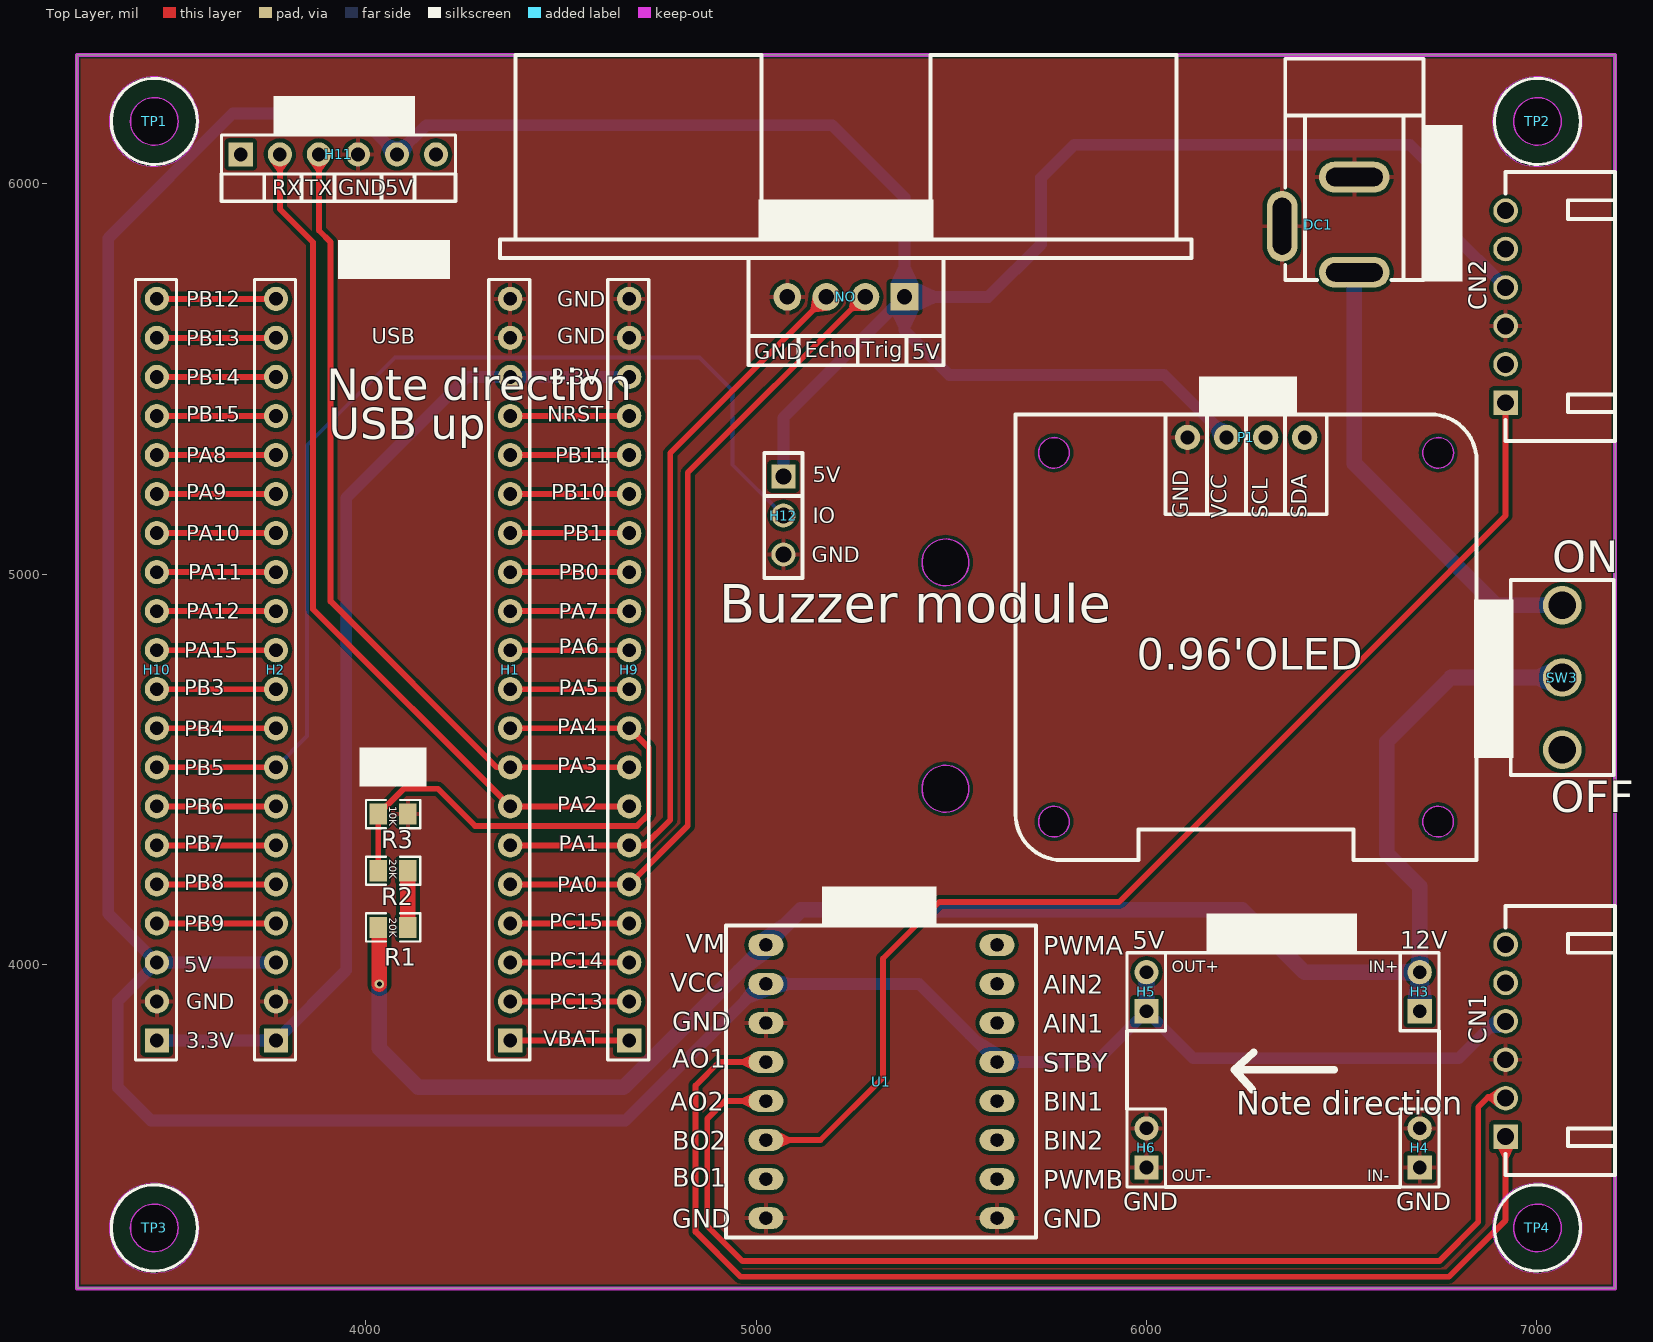
[diagram p0: Top Layer view]
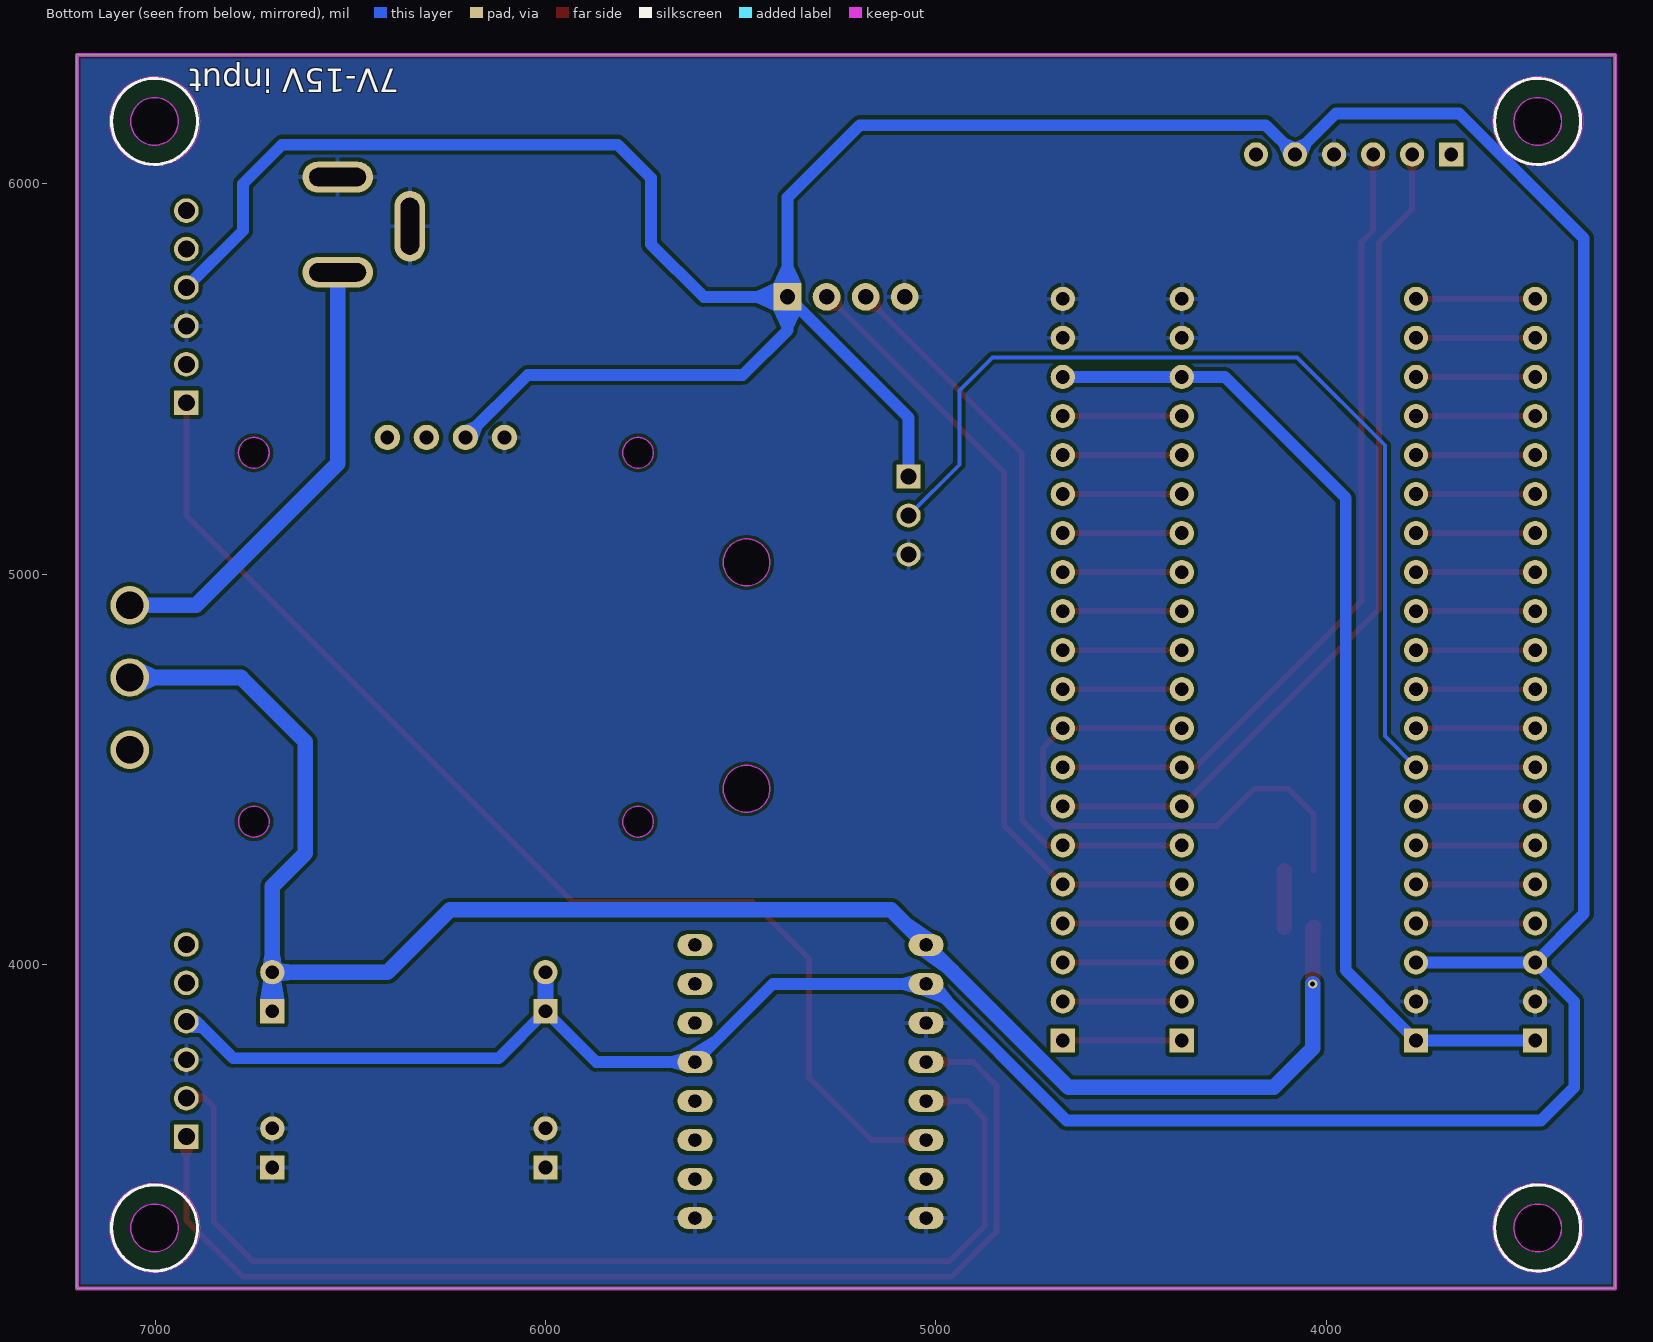
[diagram p1: Bottom Layer view, seen from below]
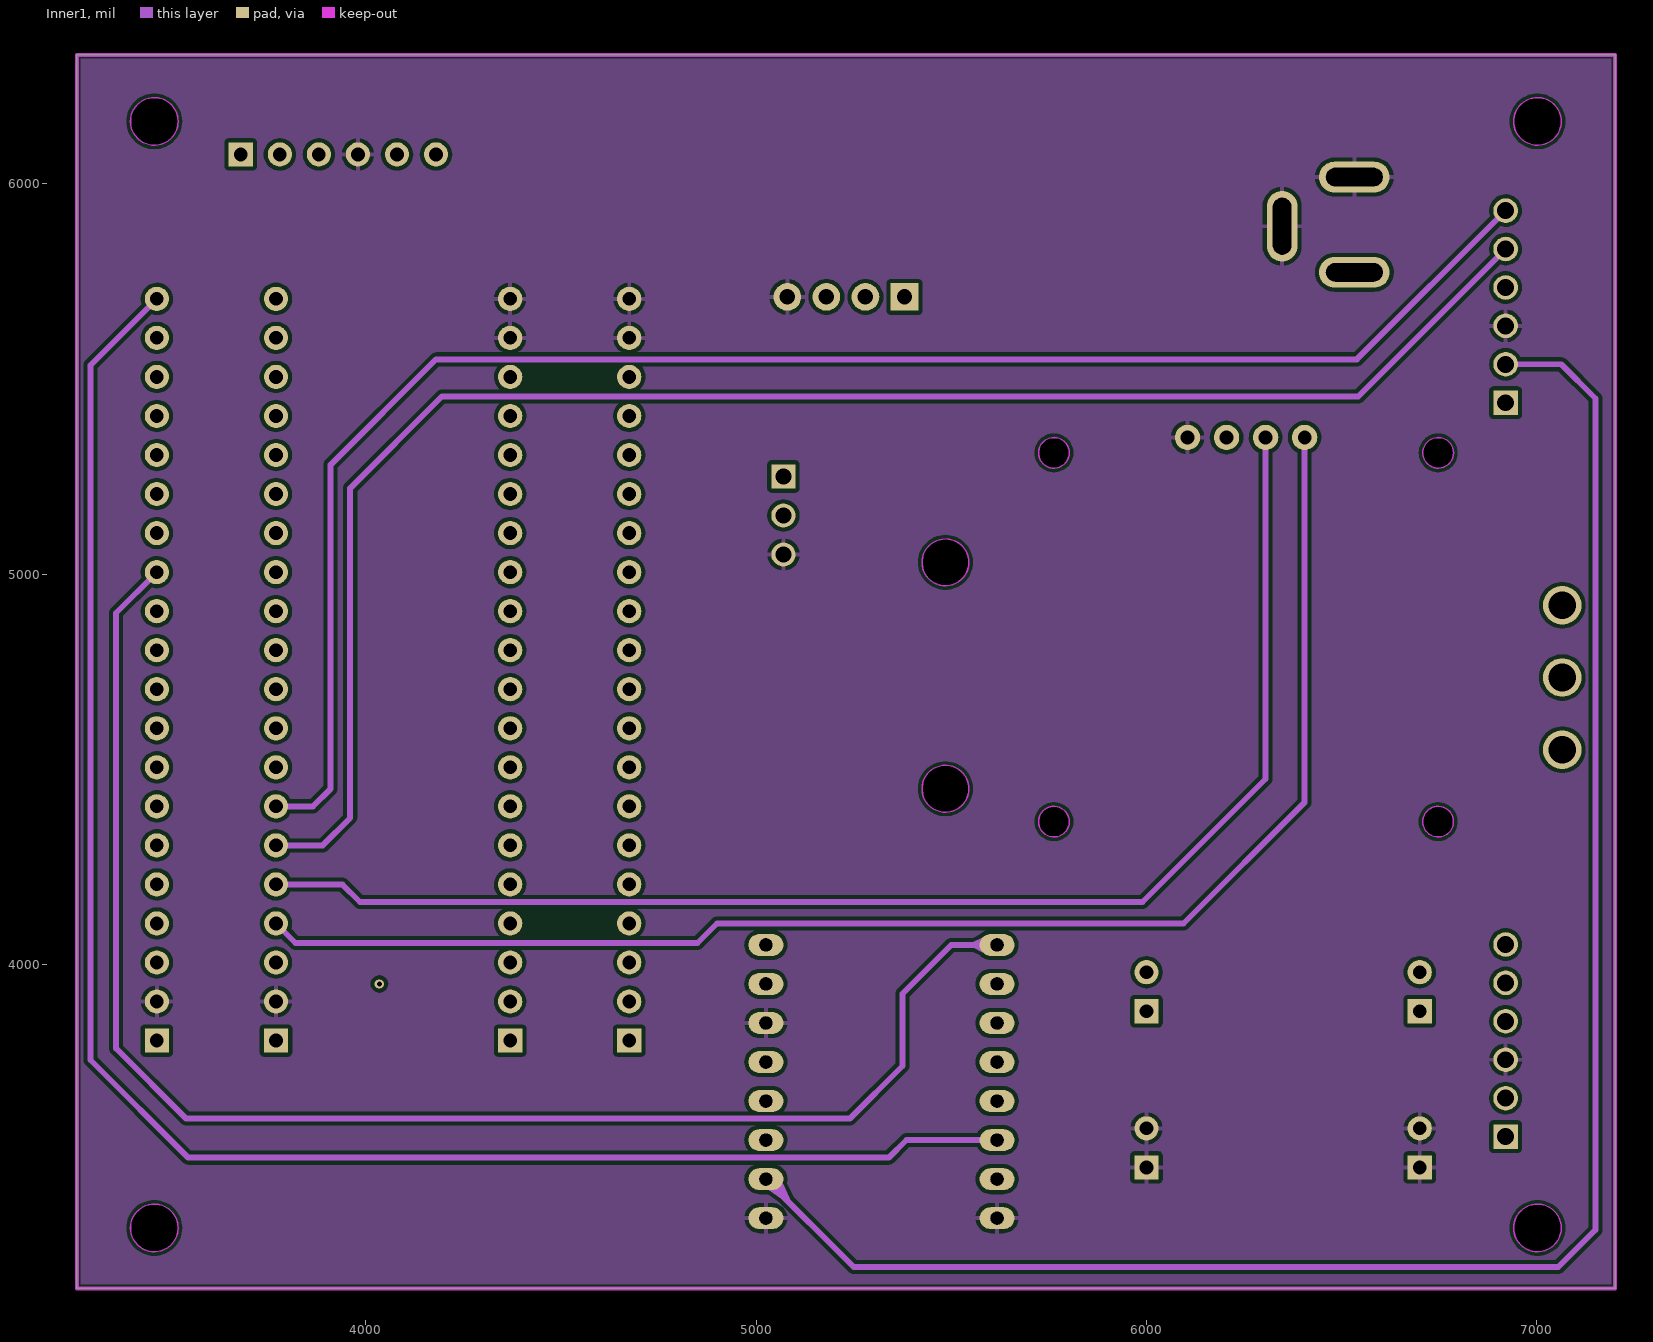
[diagram p2: Inner1]
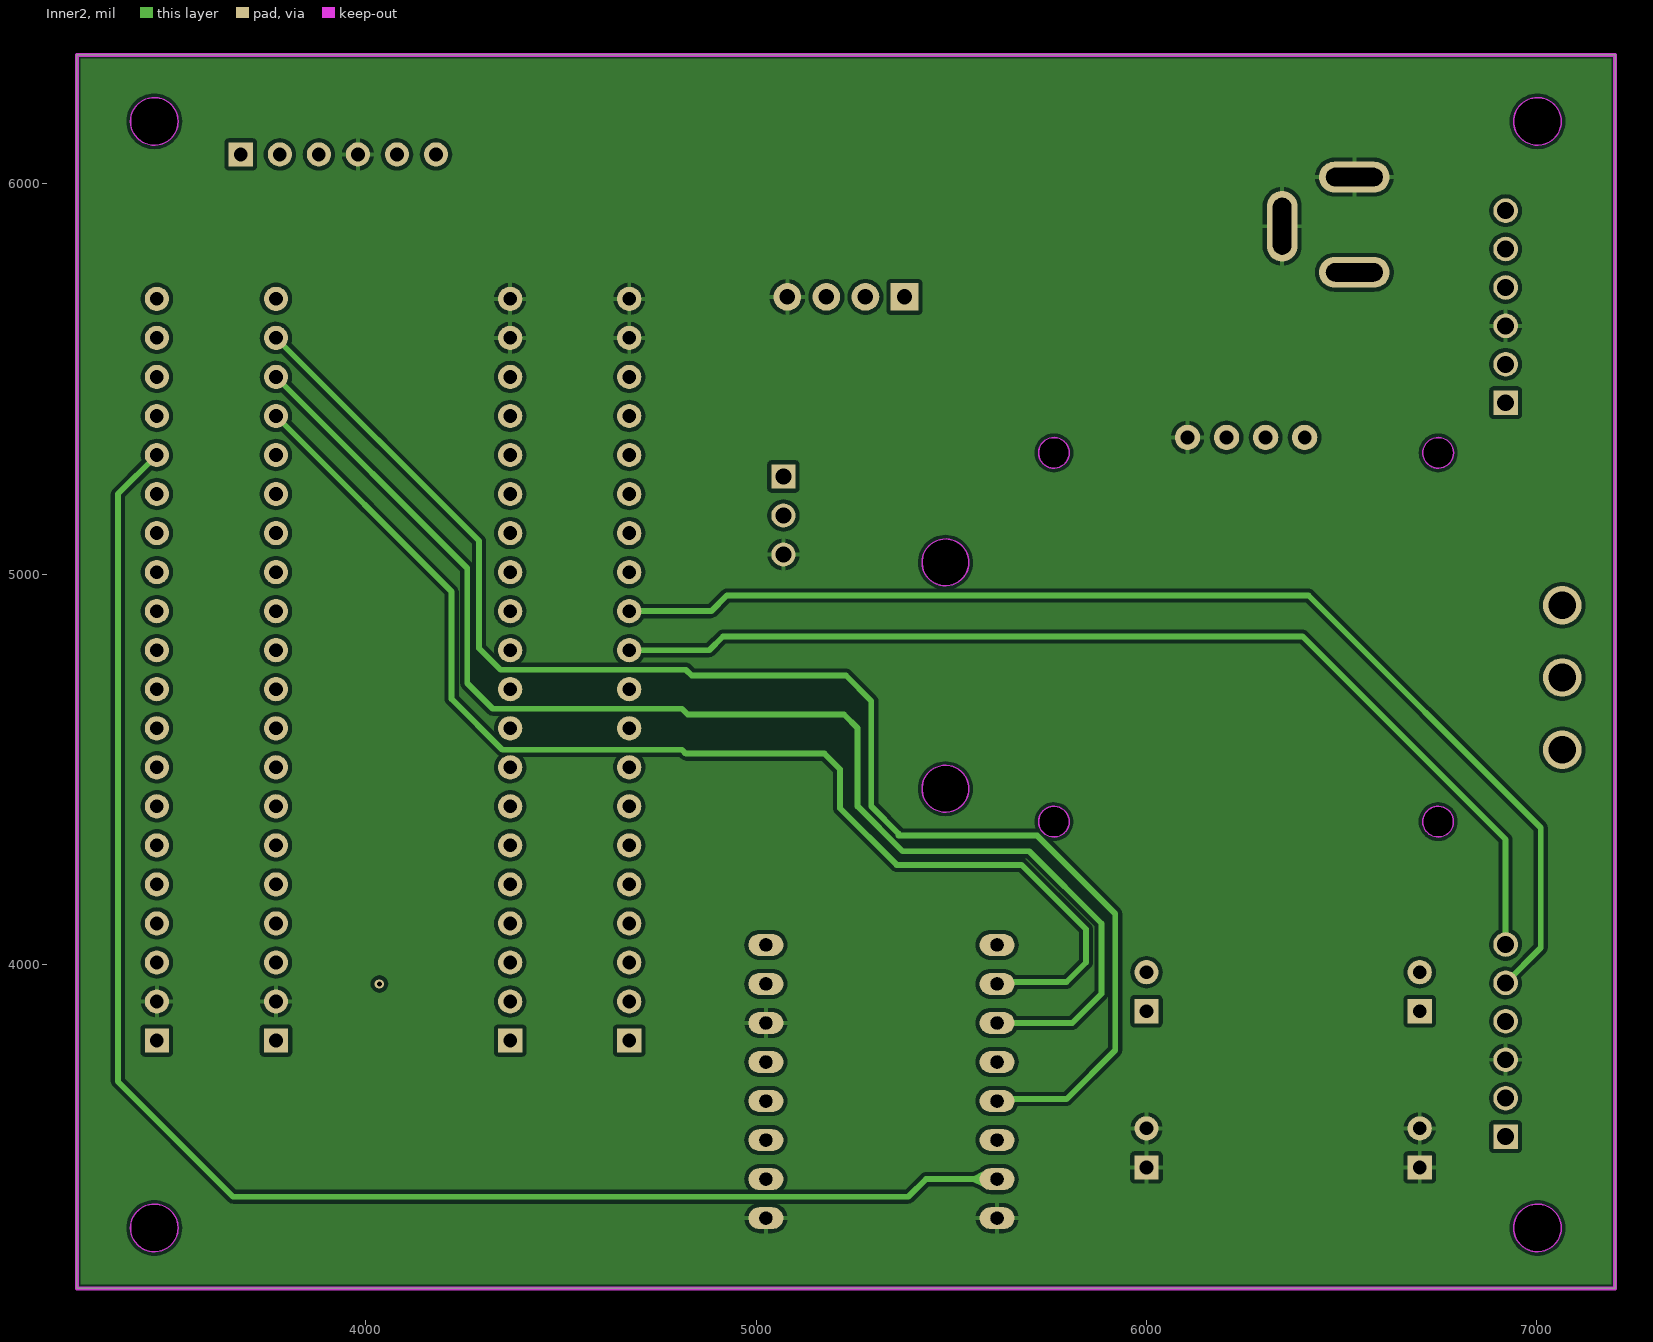
[diagram p3: Inner2]
# Altium PCB MISC51780.pcbdoc (part 1 of 2)
Units mil, origin at the board's own origin, x right, y up, seen from the top; angles counter-clockwise.
Board outline 3940.5 x 3159.99 mil, 4 copper layers (Top Layer, Inner1, Inner2, Bottom Layer), stack 62.206 mil thick; 24 components, 44 nets, 145 pads, 1 vias.

## Layer stack, top to bottom
Top Solder Mask Layer: solder mask 0.394, Dk 3.3
Top Layer: signal copper 1.378
Dielectric1: surface 18.898, PP, Dk 4.5
Inner1: signal copper 1.378
Dielectric2: surface 18.898, FR4, Dk 4.5
Inner2: signal copper 1.378
Dielectric3: surface 18.898, PP, Dk 4.5
Bottom Layer: signal copper 1.378
Bottom Solder Mask Layer: solder mask 0.394, Dk 3.3

## Board outline
3260,3170.01 3260,6330 7200.5,6330 7200.5,3170.01
cut-out: 5545,4450 cw(c5485,4450) 5425,4450 cw(c5485,4450)
cut-out: 5545,5030 cw(c5485,5030) 5425,5030 cw(c5485,5030)

## Design rules (kind name [scope] priority, off if disabled: settings)
BoardOutlineClearance Plane_innerPlane_1 [All] p2 off: genericclearance=6 ignorepadtopadclearanceinfootprint=FALSE except(0: Arc-SplitContinuation Track-SplitContinuation SMDPad-SplitContinuation THPad-SplitContinuation Via-SplitContinuation Fill-SplitContinuation Region-SplitContinuation Poly-SplitContinuation Text-SplitContinuation Hole-SplitContinuation; 6: Arc-CutoutEdge Track-CutoutEdge SMDPad-CutoutEdge THPad-CutoutEdge Via-CutoutEdge Fill-CutoutEdge Region-CutoutEdge Text-CutoutEdge; 6.9: Hole-OutlineEdge Hole-CutoutEdge; 10: Poly-OutlineEdge Poly-CutoutEdge; 11.8: Arc-OutlineEdge Track-OutlineEdge SMDPad-OutlineEdge THPad-OutlineEdge Via-OutlineEdge Fill-OutlineEdge Region-OutlineEdge Text-OutlineEdge)
BoardOutlineClearance Copper_copperRegion_1 [All] p4 off: genericclearance=6 ignorepadtopadclearanceinfootprint=FALSE except(0: Arc-SplitContinuation Track-SplitContinuation SMDPad-SplitContinuation THPad-SplitContinuation Via-SplitContinuation Fill-SplitContinuation Region-SplitContinuation Poly-SplitContinuation Text-SplitContinuation Hole-SplitContinuation; 6: Arc-CutoutEdge Track-CutoutEdge SMDPad-CutoutEdge THPad-CutoutEdge Via-CutoutEdge Fill-CutoutEdge Region-CutoutEdge Text-CutoutEdge; 6.9: Hole-OutlineEdge Hole-CutoutEdge; 10: Poly-OutlineEdge Poly-CutoutEdge; 11.8: Arc-OutlineEdge Track-OutlineEdge SMDPad-OutlineEdge THPad-OutlineEdge Via-OutlineEdge Fill-OutlineEdge Region-OutlineEdge Text-OutlineEdge)
BoardOutlineClearance Copper_gge61610_1 [All] p6 off: genericclearance=6 ignorepadtopadclearanceinfootprint=FALSE except(0: Arc-SplitContinuation Track-SplitContinuation SMDPad-SplitContinuation THPad-SplitContinuation Via-SplitContinuation Fill-SplitContinuation Region-SplitContinuation Poly-SplitContinuation Text-SplitContinuation Hole-SplitContinuation; 6: Arc-CutoutEdge Track-CutoutEdge SMDPad-CutoutEdge THPad-CutoutEdge Via-CutoutEdge Fill-CutoutEdge Region-CutoutEdge Text-CutoutEdge; 6.9: Hole-OutlineEdge Hole-CutoutEdge; 10: Poly-OutlineEdge Poly-CutoutEdge; 11.8: Arc-OutlineEdge Track-OutlineEdge SMDPad-OutlineEdge THPad-OutlineEdge Via-OutlineEdge Fill-OutlineEdge Region-OutlineEdge Text-OutlineEdge)
BoardOutlineClearance Copper_gge61631_1 [All] p8 off: genericclearance=6 ignorepadtopadclearanceinfootprint=FALSE except(0: Arc-SplitContinuation Track-SplitContinuation SMDPad-SplitContinuation THPad-SplitContinuation Via-SplitContinuation Fill-SplitContinuation Region-SplitContinuation Poly-SplitContinuation Text-SplitContinuation Hole-SplitContinuation; 6: Arc-CutoutEdge Track-CutoutEdge SMDPad-CutoutEdge THPad-CutoutEdge Via-CutoutEdge Fill-CutoutEdge Region-CutoutEdge Text-CutoutEdge; 6.9: Hole-OutlineEdge Hole-CutoutEdge; 10: Poly-OutlineEdge Poly-CutoutEdge; 11.8: Arc-OutlineEdge Track-OutlineEdge SMDPad-OutlineEdge THPad-OutlineEdge Via-OutlineEdge Fill-OutlineEdge Region-OutlineEdge Text-OutlineEdge)
BoardOutlineClearance Copper_gge61637_1 [All] p10 off: genericclearance=6 ignorepadtopadclearanceinfootprint=FALSE except(0: Arc-SplitContinuation Track-SplitContinuation SMDPad-SplitContinuation THPad-SplitContinuation Via-SplitContinuation Fill-SplitContinuation Region-SplitContinuation Poly-SplitContinuation Text-SplitContinuation Hole-SplitContinuation; 6: Arc-CutoutEdge Track-CutoutEdge SMDPad-CutoutEdge THPad-CutoutEdge Via-CutoutEdge Fill-CutoutEdge Region-CutoutEdge Text-CutoutEdge; 6.9: Hole-OutlineEdge Hole-CutoutEdge; 10: Poly-OutlineEdge Poly-CutoutEdge; 11.8: Arc-OutlineEdge Track-OutlineEdge SMDPad-OutlineEdge THPad-OutlineEdge Via-OutlineEdge Fill-OutlineEdge Region-OutlineEdge Text-OutlineEdge)
BoardOutlineClearance Copper_gge61622(1)_1 [All] p12 off: genericclearance=6 ignorepadtopadclearanceinfootprint=FALSE except(0: Arc-SplitContinuation Track-SplitContinuation SMDPad-SplitContinuation THPad-SplitContinuation Via-SplitContinuation Fill-SplitContinuation Region-SplitContinuation Poly-SplitContinuation Text-SplitContinuation Hole-SplitContinuation; 6: Arc-CutoutEdge Track-CutoutEdge SMDPad-CutoutEdge THPad-CutoutEdge Via-CutoutEdge Fill-CutoutEdge Region-CutoutEdge Text-CutoutEdge; 6.9: Hole-OutlineEdge Hole-CutoutEdge; 10: Poly-OutlineEdge Poly-CutoutEdge; 11.8: Arc-OutlineEdge Track-OutlineEdge SMDPad-OutlineEdge THPad-OutlineEdge Via-OutlineEdge Fill-OutlineEdge Region-OutlineEdge Text-OutlineEdge)
BoardOutlineClearance safeClearance_1 [All] p14: genericclearance=6 ignorepadtopadclearanceinfootprint=FALSE except(0: Arc-SplitContinuation Track-SplitContinuation SMDPad-SplitContinuation THPad-SplitContinuation Via-SplitContinuation Fill-SplitContinuation Region-SplitContinuation Poly-SplitContinuation Text-SplitContinuation Hole-SplitContinuation; 6: Arc-CutoutEdge Track-CutoutEdge SMDPad-CutoutEdge THPad-CutoutEdge Via-CutoutEdge Fill-CutoutEdge Region-CutoutEdge Text-CutoutEdge; 6.9: Hole-OutlineEdge Hole-CutoutEdge; 10: Poly-OutlineEdge Poly-CutoutEdge; 11.8: Arc-OutlineEdge Track-OutlineEdge SMDPad-OutlineEdge THPad-OutlineEdge Via-OutlineEdge Fill-OutlineEdge Region-OutlineEdge Text-OutlineEdge)
Clearance Plane_innerPlane [All] p1 off: gap=6 ignorepadtopadclearanceinfootprint=FALSE except(6.9: Hole-Track Hole-SMDPad Hole-THPad Hole-Via Fill-Hole Region-Hole Hole-Arc Hole-Text; 10: Poly-Track Poly-SMDPad Poly-THPad Poly-Via Poly-Fill Poly-Region Poly-Poly Poly-Arc Poly-Text Poly-Hole)
Clearance Copper_copperRegion [All] p3 off: gap=6 ignorepadtopadclearanceinfootprint=FALSE except(6.9: Hole-Track Hole-SMDPad Hole-THPad Hole-Via Fill-Hole Region-Hole Hole-Arc Hole-Text; 10: Poly-Track Poly-SMDPad Poly-THPad Poly-Via Poly-Fill Poly-Region Poly-Poly Poly-Arc Poly-Text Poly-Hole)
Clearance Copper_gge61610 [All] p5 off: gap=6 ignorepadtopadclearanceinfootprint=FALSE except(6.9: Hole-Track Hole-SMDPad Hole-THPad Hole-Via Fill-Hole Region-Hole Hole-Arc Hole-Text; 10: Poly-Track Poly-SMDPad Poly-THPad Poly-Via Poly-Fill Poly-Region Poly-Poly Poly-Arc Poly-Text Poly-Hole)
Clearance Copper_gge61631 [All] p7 off: gap=6 ignorepadtopadclearanceinfootprint=FALSE except(6.9: Hole-Track Hole-SMDPad Hole-THPad Hole-Via Fill-Hole Region-Hole Hole-Arc Hole-Text; 10: Poly-Track Poly-SMDPad Poly-THPad Poly-Via Poly-Fill Poly-Region Poly-Poly Poly-Arc Poly-Text Poly-Hole)
Clearance Copper_gge61637 [All] p9 off: gap=6 ignorepadtopadclearanceinfootprint=FALSE except(6.9: Hole-Track Hole-SMDPad Hole-THPad Hole-Via Fill-Hole Region-Hole Hole-Arc Hole-Text; 10: Poly-Track Poly-SMDPad Poly-THPad Poly-Via Poly-Fill Poly-Region Poly-Poly Poly-Arc Poly-Text Poly-Hole)
Clearance Copper_gge61622(1) [All] p11 off: gap=6 ignorepadtopadclearanceinfootprint=FALSE except(6.9: Hole-Track Hole-SMDPad Hole-THPad Hole-Via Fill-Hole Region-Hole Hole-Arc Hole-Text; 10: Poly-Track Poly-SMDPad Poly-THPad Poly-Via Poly-Fill Poly-Region Poly-Poly Poly-Arc Poly-Text Poly-Hole)
Clearance safeClearance [All] p13: gap=6 ignorepadtopadclearanceinfootprint=FALSE except(6.9: Hole-Track Hole-SMDPad Hole-THPad Hole-Via Fill-Hole Region-Hole Hole-Arc Hole-Text; 10: Poly-Track Poly-SMDPad Poly-THPad Poly-Via Poly-Fill Poly-Region Poly-Poly Poly-Arc Poly-Text Poly-Hole)
DiffPairsRouting differentialPair [All] p1: maxlimit=6 minlimit=6 mostfreqgap=6 toplayer_minwidth=5 toplayer_prefwidth=10 toplayer_maxwidth=100 toplayer_mingap=6 toplayer_prefgap=6 toplayer_maxgap=6 midlayer1_minwidth=5 midlayer1_prefwidth=10 midlayer1_maxwidth=100 midlayer1_mingap=6 midlayer1_prefgap=6 midlayer1_maxgap=6 midlayer2_minwidth=5 midlayer2_prefwidth=10 midlayer2_maxwidth=100 midlayer2_mingap=6 midlayer2_prefgap=6 midlayer2_maxgap=6 bottomlayer_minwidth=5 bottomlayer_prefwidth=10 bottomlayer_maxwidth=100 bottomlayer_mingap=6 bottomlayer_prefgap=6 bottomlayer_maxgap=6 maxuncoupledlength=10
HoleToHoleClearance gge61610 [All] p1 off: gap=0 allowstackedmicrovias=TRUE
HoleToHoleClearance gge61631 [All] p2 off: gap=0 allowstackedmicrovias=TRUE
HoleToHoleClearance gge61637 [All] p3 off: gap=0 allowstackedmicrovias=TRUE
HoleToHoleClearance gge61622 [All] p4 off: gap=0 allowstackedmicrovias=TRUE
HoleToHoleClearance gge61622(1) [All] p5 off: gap=0 allowstackedmicrovias=TRUE
HoleToHoleClearance Common [All] p6: gap=11.8 allowstackedmicrovias=TRUE
Length netLength [All] p1: minlimit=0 maxlimit=0
PasteMaskExpansion pasteMaskExpansion [All] p1: expansion=0
PlaneConnect innerPlane [All] p1: planeconnectstyle=Relief reliefexpansion=20 reliefentries=4 reliefconductorwidth=10 reliefairgap=10
PolygonConnect gge61610_1 [All] p1 off: connectstyle=Relief reliefconductorwidth=10 reliefentries=4 polygonreliefangle="90 Angle" airgapwidth=10 via.connectstyle=Relief via.reliefconductorwidth=10 via.reliefentries=4 via.polygonreliefangle="90 Angle" via.airgapwidth=10
PolygonConnect gge61631_1 [All] p2 off: connectstyle=Relief reliefconductorwidth=10 reliefentries=4 polygonreliefangle="90 Angle" airgapwidth=10 via.connectstyle=Relief via.reliefconductorwidth=10 via.reliefentries=4 via.polygonreliefangle="90 Angle" via.airgapwidth=10
PolygonConnect gge61637_1 [All] p3 off: connectstyle=Relief reliefconductorwidth=10 reliefentries=4 polygonreliefangle="90 Angle" airgapwidth=10 via.connectstyle=Relief via.reliefconductorwidth=10 via.reliefentries=4 via.polygonreliefangle="90 Angle" via.airgapwidth=10
PolygonConnect gge61622(1)_1 [All] p4 off: connectstyle=Relief reliefconductorwidth=10 reliefentries=4 polygonreliefangle="90 Angle" airgapwidth=10 via.connectstyle=Relief via.reliefconductorwidth=10 via.reliefentries=4 via.polygonreliefangle="90 Angle" via.airgapwidth=10
PolygonConnect copperRegion [All] p5: connectstyle=Relief reliefconductorwidth=10 reliefentries=4 polygonreliefangle="90 Angle" airgapwidth=10 via.connectstyle=Relief via.reliefconductorwidth=10 via.reliefentries=4 via.polygonreliefangle="90 Angle" via.airgapwidth=10
RoutingVias viaSize [All] p1: holewidth=12.01 width=24.02 viastyle="Through Hole" minholewidth=11.81 minwidth=19.68 maxholewidth=236.22 maxwidth=393.7
SolderMaskExpansion solderMaskExpansion [IsVia] p1: expansion=-1000 istentingtop=TRUE
SolderMaskExpansion solderMaskExpansion [All] p2: expansion=2 istentingtop=FALSE
Width trackWidth [All] p1: maxlimit=100 minlimit=5 preferedwidth=10

## Components (designator, comment, footprint, x,y, rotation, side; value= is the part's Value field where it differs from the comment)
CN1 "MOTO1" CONN-TH_6P-P2.50_X8821WR-06S-N2SN 6920,3805 r90 top locked
CN2 "MOTO2" CONN-TH_6P-P2.50_X8821WR-06S-N2SN 6920,5685 r90 top
DC1 "DC005_C431533" DC-IN-TH_DC005 6440,5895 r270 top
H1 "HDR-F-2.54_1x20" HDR-F-2.54_1X20 4370,4755 r90 top
H2 "HDR-F-2.54_1x20" HDR-F-2.54_1X20 3770,4755 r90 top
H3 "HDR-F-2.54_1x2" HDR-F-2.54_1X2 6700,3930 r90 top
H4 "HDR-F-2.54_1x2" HDR-F-2.54_1X2 6700,3530 r90 top
H5 "HDR-F-2.54_1x2" HDR-F-2.54_1X2 6000,3930 r90 top
H6 "HDR-F-2.54_1x2" HDR-F-2.54_1X2 6000,3530 r90 top
H9 "HDR-F-2.54_1x20" HDR-F-2.54_1X20 4675,4755 r90 top
H10 "HDR-F-2.54_1x20" HDR-F-2.54_1X20 3465,4755 r90 top
H11 "Bluetooth" HDR-F-2.54_1X6 3880,6075 r0 top
H12 "" HDR-TH_3P-P2.54-V-F 5070,5150 r270 top
NO "MODULE_HC-SR04" HC-SR04 5230,5710 r180 top
P1 "0.96OLED_4P" 0.96OLED_4P 6255,5350 r0 top
R1 "20K" R0805 4070,4095 r180 top
R2 "20K" R0805 4070,4240 r0 top
R3 "10K" R0805 4070,4385 r180 top
SW3 "SS-12D10L5" SW-TH_SS-12D10L5 7065,4735 r270 top
TP1 "M3 standoff with silkscreen" M3铜柱 3458.27,6159.65 r0 top locked
TP2 "M3 standoff with silkscreen" M3铜柱 7001.57,6159.65 r0 top
TP3 "M3 standoff with silkscreen" M3铜柱 3458.27,3325 r0 top
TP4 "M3 standoff with silkscreen" M3铜柱 7001.57,3325 r0 top
U1 "TB6612FNG component" TB6612FNG封装 5320,3700 r0 top

## Footprints (in the part's own frame and the unit in brackets; to place one, negate y for a bottom-side part, rotate by r counter-clockwise, add the part's x,y. Pads: shape width x height; smd on the part's side, far side on the other; paste and mask are expansions set on the pad)
0.96OLED_4P [mm]
  round 1.65 hole 0.89 paste+0 mask+0.102: 1(-3.807,-0.003) 2(-1.267,0) 3(1.273,0) 4(3.813,0)
  Board Outline Layer circle w0.003: c-12.499,-1.001 r1
  Board Outline Layer circle w0.003: c12.502,-1.001 r1
  Board Outline Layer circle w0.003: c12.499,-25.001 r1
  Board Outline Layer circle w0.003: c-12.499,-25.001 r1
  Board Outline Layer region: -11.499,-1.001 -11.598,-1.435 -11.876,-1.783 -12.277,-1.976 -12.722,-1.976 -13.123,-1.783 -13.4,-1.435 -13.499,-1.001 -13.499,-1.001 -13.4,-0.567 -13.123,-0.219 -12.722,-0.026 -12.277,-0.026 -11.876,-0.219 -11.598,-0.567 -11.499,-1.001
  Board Outline Layer region: -11.499,-1.001 -11.509,-1.137 -11.536,-1.271 -11.582,-1.399 -11.645,-1.52 -11.724,-1.632 -11.817,-1.732 -11.923,-1.818 -12.039,-1.889 -12.164,-1.943 -12.296,-1.98 -12.431,-1.998 -12.568,-1.998 -12.703,-1.98 -12.834,-1.943 -12.959,-1.889 -13.076,-1.818 -13.182,-1.732 -13.275,-1.632 -13.354,-1.52 -13.417,-1.399 -13.462,-1.271 -13.49,-1.137 -13.499,-1.001 -13.49,-0.865 -13.462,-0.731 -13.417,-0.602 -13.354,-0.481 -13.275,-0.37 -13.182,-0.27 -13.076,-0.184 -12.959,-0.113 -12.834,-0.059 -12.703,-0.022 -12.568,-0.003 -12.431,-0.003 -12.296,-0.022 -12.164,-0.059 -12.039,-0.113 -11.923,-0.184 -11.817,-0.27 -11.724,-0.37 -11.645,-0.481 -11.582,-0.602 -11.536,-0.731 -11.509,-0.865
  Board Outline Layer region: 13.502,-1.001 13.403,-1.435 13.125,-1.783 12.724,-1.976 12.279,-1.976 11.878,-1.783 11.601,-1.435 11.502,-1.001 11.502,-1.001 11.601,-0.567 11.878,-0.219 12.279,-0.026 12.724,-0.026 13.125,-0.219 13.403,-0.567 13.502,-1.001
  Board Outline Layer region: 13.502,-1.001 13.493,-1.137 13.465,-1.271 13.419,-1.399 13.356,-1.52 13.278,-1.632 13.184,-1.732 13.079,-1.818 12.962,-1.889 12.837,-1.943 12.705,-1.98 12.57,-1.998 12.434,-1.998 12.298,-1.98 12.167,-1.943 12.042,-1.889 11.925,-1.818 11.819,-1.732 11.726,-1.632 11.647,-1.52 11.585,-1.399 11.539,-1.271 11.511,-1.137 11.502,-1.001 11.511,-0.865 11.539,-0.731 11.585,-0.602 11.647,-0.481 11.726,-0.37 11.819,-0.27 11.925,-0.184 12.042,-0.113 12.167,-0.059 12.298,-0.022 12.434,-0.003 12.57,-0.003 12.705,-0.022 12.837,-0.059 12.962,-0.113 13.079,-0.184 13.184,-0.27 13.278,-0.37 13.356,-0.481 13.419,-0.602 13.465,-0.731 13.493,-0.865
  Board Outline Layer region: 13.499,-25.001 13.4,-25.435 13.123,-25.783 12.722,-25.976 12.277,-25.976 11.876,-25.783 11.598,-25.435 11.499,-25.001 11.499,-25.001 11.598,-24.567 11.876,-24.219 12.277,-24.026 12.722,-24.026 13.123,-24.219 13.4,-24.567 13.499,-25.001
  Board Outline Layer region: 13.499,-25.001 13.49,-25.137 13.462,-25.271 13.417,-25.4 13.354,-25.521 13.275,-25.632 13.182,-25.732 13.076,-25.818 12.959,-25.889 12.834,-25.943 12.703,-25.98 12.568,-25.999 12.431,-25.999 12.296,-25.98 12.164,-25.943 12.039,-25.889 11.923,-25.818 11.817,-25.732 11.724,-25.632 11.645,-25.521 11.582,-25.4 11.536,-25.271 11.509,-25.137 11.499,-25.001 11.509,-24.865 11.536,-24.731 11.582,-24.603 11.645,-24.482 11.724,-24.37 11.817,-24.27 11.923,-24.184 12.039,-24.113 12.164,-24.059 12.296,-24.022 12.431,-24.004 12.568,-24.004 12.703,-24.022 12.834,-24.059 12.959,-24.113 13.076,-24.184 13.182,-24.27 13.275,-24.37 13.354,-24.482 13.417,-24.603 13.462,-24.731 13.49,-24.865
  Board Outline Layer region: -11.499,-25.001 -11.598,-25.435 -11.876,-25.783 -12.277,-25.976 -12.722,-25.976 -13.123,-25.783 -13.4,-25.435 -13.499,-25.001 -13.499,-25.001 -13.4,-24.567 -13.123,-24.219 -12.722,-24.026 -12.277,-24.026 -11.876,-24.219 -11.598,-24.567 -11.499,-25.001
  Board Outline Layer region: -11.499,-25.001 -11.509,-25.137 -11.536,-25.271 -11.582,-25.4 -11.645,-25.521 -11.724,-25.632 -11.817,-25.732 -11.923,-25.818 -12.039,-25.889 -12.164,-25.943 -12.296,-25.98 -12.431,-25.999 -12.568,-25.999 -12.703,-25.98 -12.834,-25.943 -12.959,-25.889 -13.076,-25.818 -13.182,-25.732 -13.275,-25.632 -13.354,-25.521 -13.417,-25.4 -13.462,-25.271 -13.49,-25.137 -13.499,-25.001 -13.49,-24.865 -13.462,-24.731 -13.417,-24.603 -13.354,-24.482 -13.275,-24.37 -13.182,-24.27 -13.076,-24.184 -12.959,-24.113 -12.834,-24.059 -12.703,-24.022 -12.568,-24.004 -12.431,-24.004 -12.296,-24.022 -12.164,-24.059 -12.039,-24.113 -11.923,-24.184 -11.817,-24.27 -11.724,-24.37 -11.645,-24.482 -11.582,-24.603 -11.536,-24.731 -11.509,-24.865
  Multi-Layer board cut-out: -11.499,-1.001 -11.598,-1.435 -11.876,-1.783 -12.277,-1.976 -12.722,-1.976 -13.123,-1.783 -13.4,-1.435 -13.499,-1.001 -13.499,-1.001 -13.4,-0.567 -13.123,-0.219 -12.722,-0.026 -12.277,-0.026 -11.876,-0.219 -11.598,-0.567 -11.499,-1.001
  Multi-Layer board cut-out: 13.502,-1.001 13.403,-1.435 13.125,-1.783 12.724,-1.976 12.279,-1.976 11.878,-1.783 11.601,-1.435 11.502,-1.001 11.502,-1.001 11.601,-0.567 11.878,-0.219 12.279,-0.026 12.724,-0.026 13.125,-0.219 13.403,-0.567 13.502,-1.001
  Multi-Layer board cut-out: 13.499,-25.001 13.4,-25.435 13.123,-25.783 12.722,-25.976 12.277,-25.976 11.876,-25.783 11.598,-25.435 11.499,-25.001 11.499,-25.001 11.598,-24.567 11.876,-24.219 12.277,-24.026 12.722,-24.026 13.123,-24.219 13.4,-24.567 13.499,-25.001
  Multi-Layer board cut-out: -11.499,-25.001 -11.598,-25.435 -11.876,-25.783 -12.277,-25.976 -12.722,-25.976 -13.123,-25.783 -13.4,-25.435 -13.499,-25.001 -13.499,-25.001 -13.4,-24.567 -13.123,-24.219 -12.722,-24.026 -12.277,-24.026 -11.876,-24.219 -11.598,-24.567 -11.499,-25.001
  silkscreen extent -15,-27.5 15,1.5
CONN-TH_6P-P2.50_X8821WR-06S-N2SN [mm]
  rect 1.6x1.6 hole 1.1: 1(-6.25,0)
  round 1.6 hole 1.1: 2(-3.75,0) 3(-1.25,0) 4(1.25,0) 5(3.75,0) 6(6.25,0)
  silkscreen extent -8.75,-7.11 8.75,0
DC-IN-TH_DC005 [mm]
  oval 2x4.6 hole 1.2 slot 3.7 at 90 deg: 1(3.1,2.35) 2(-3.1,2.35)
  oval 4.6x2 hole 1.2 slot 3.7 at 0 deg: 3(0.1,-2.35)
  silkscreen extent -10.8,-2.15 3.6,6.85
HC-SR04 [mm]
  rect 1.8x1.8 hole 1 paste+0 mask+0.102: 1(-3.81,0)
  round 1.8 hole 1 paste+0 mask+0.102: 2(-1.27,0) 3(1.27,0) 4(3.81,0)
  silkscreen extent -22.5,-15.74 22.5,2.54
HDR-F-2.54_1X2 [mil]
  rect 62x62 hole 35: 1(-50,0)
  round 62 hole 35: 2(50,0)
  silkscreen extent -100,-49 100,50
HDR-F-2.54_1X6 [mil]
  rect 62x62 hole 35: 1(-200,0)
  round 62 hole 35: 2(-100,0) 3(0,0) 4(100,0) 5(200,0) 6(300,0)
  silkscreen extent -250,-50 350,50
HDR-F-2.54_1X20 [mil]
  rect 62x62 hole 35: 1(-950,0)
  round 62 hole 35: 2(-850,0) 3(-750,0) 4(-650,0) 5(-550,0) 6(-450,0) 7(-350,0) 8(-250,0) 9(-150,0) 10(-50,0) 11(50,0) 12(150,0) 13(250,0) 14(350,0) 15(450,0) 16(550,0) 17(650,0) 18(750,0) 19(850,0) 20(950,0)
  silkscreen extent -1000,-50 1000,55
HDR-TH_3P-P2.54-V-F [mil]
  rect 62x62 hole 40.16: 1(-100,0)
  round 62 hole 40.16: 2(0,0) 3(100,0)
  silkscreen extent -160,-49 160,49
M3铜柱 [mil]
  Top Layer keep-out region: -0.35,-115.47 9.15,-115.07 18.59,-113.89 27.9,-111.94 37.01,-109.22 45.87,-105.76 54.41,-101.58 62.58,-96.71 70.32,-91.18 77.57,-85.03 84.29,-78.31 90.44,-71.05 95.96,-63.31 100.83,-55.14 105,-46.59 108.45,-37.73 111.17,-28.62 113.12,-19.31 114.29,-9.87 114.68,-0.37 114.29,9.13 113.11,18.57 111.15,27.88 108.44,36.99 104.98,45.85 100.8,54.39 95.93,62.56 90.41,70.3 84.26,77.55 77.53,84.28 70.28,90.42 62.54,95.95 54.37,100.82 45.82,104.99 36.96,108.45 27.85,111.16 18.54,113.11 9.1,114.29 -0.4,114.68 -9.9,114.29 -19.34,113.11 -28.64,111.16 -37.76,108.45 -46.62,104.99 -55.16,100.82 -63.33,95.95 -71.07,90.42 -78.33,84.28 -85.05,77.55 -91.2,70.3 -96.73,62.56 -101.6,54.39 -105.77,45.85 -109.23,36.99 -111.95,27.88 -113.9,18.57 -115.08,9.13 -115.47,-0.37 -115.08,-9.87 -113.91,-19.31 -111.96,-28.62 -109.25,-37.73 -105.79,-46.59 -101.62,-55.14 -96.75,-63.31 -91.23,-71.05 -85.09,-78.31 -78.36,-85.03 -71.11,-91.18 -63.37,-96.71 -55.2,-101.58 -46.66,-105.76 -37.8,-109.22 -28.69,-111.94 -19.38,-113.89 -9.95,-115.07 -0.45,-115.47 -0.35,-115.47
  Bottom Layer keep-out region: -0.34,-114.68 9.16,-114.29 18.59,-113.11 27.9,-111.15 37.01,-108.43 45.87,-104.97 54.41,-100.79 62.58,-95.92 70.32,-90.39 77.57,-84.24 84.29,-77.52 90.44,-70.26 95.96,-62.52 100.83,-54.35 105,-45.8 108.46,-36.94 111.17,-27.83 113.12,-18.52 114.29,-9.08 114.68,0.42 114.29,9.92 113.11,19.36 111.16,28.66 108.44,37.78 104.98,46.64 100.8,55.18 95.93,63.35 90.41,71.09 84.26,78.34 77.54,85.07 70.28,91.21 62.54,96.74 54.37,101.61 45.82,105.78 36.96,109.24 27.85,111.95 18.54,113.9 9.11,115.08 -0.4,115.47 -9.9,115.08 -19.33,113.9 -28.64,111.95 -37.76,109.24 -46.62,105.78 -55.16,101.61 -63.33,96.74 -71.07,91.21 -78.33,85.07 -85.05,78.34 -91.2,71.09 -96.73,63.35 -101.59,55.18 -105.77,46.64 -109.23,37.78 -111.95,28.66 -113.9,19.36 -115.08,9.92 -115.47,0.42 -115.08,-9.08 -113.91,-18.52 -111.96,-27.83 -109.25,-36.94 -105.79,-45.8 -101.62,-54.35 -96.75,-62.52 -91.23,-70.26 -85.09,-77.52 -78.36,-84.24 -71.11,-90.39 -63.37,-95.92 -55.2,-100.79 -46.66,-104.97 -37.8,-108.43 -28.69,-111.15 -19.38,-113.11 -9.95,-114.29 -0.45,-114.68 -0.34,-114.68
  Board Outline Layer circle w0.1: c0,-0.01 r61.02
  Board Outline Layer region: 61.03,-0.01 54.98,-26.48 38.05,-47.72 13.58,-59.5 -13.58,-59.5 -38.04,-47.72 -54.98,-26.48 -61.02,-0.01 -61.02,-0.01 -54.98,26.47 -38.04,47.7 -13.58,59.49 13.58,59.49 38.05,47.7 54.98,26.47 61.03,-0.01
  Board Outline Layer region: 61.03,-0.01 60.64,-6.84 59.5,-13.59 57.6,-20.16 54.98,-26.48 51.67,-32.47 47.71,-38.05 43.15,-43.16 38.05,-47.72 32.47,-51.68 26.48,-54.99 20.16,-57.61 13.58,-59.5 6.84,-60.65 0,-61.03 -6.83,-60.65 -13.58,-59.5 -20.15,-57.61 -26.47,-54.99 -32.46,-51.68 -38.04,-47.72 -43.15,-43.16 -47.71,-38.05 -51.67,-32.47 -54.98,-26.48 -57.6,-20.16 -59.49,-13.59 -60.64,-6.84 -61.02,-0.01 -60.64,6.83 -59.49,13.57 -57.6,20.15 -54.98,26.47 -51.67,32.46 -47.71,38.04 -43.15,43.14 -38.04,47.7 -32.46,51.66 -26.47,54.97 -20.15,57.59 -13.58,59.49 -6.83,60.63 0,61.02 6.84,60.63 13.58,59.49 20.16,57.59 26.48,54.97 32.47,51.66 38.05,47.7 43.15,43.14 47.71,38.04 51.67,32.46 54.98,26.47 57.6,20.15 59.5,13.57 60.64,6.83
  Multi-Layer board cut-out: 61.03,-0.01 54.98,-26.48 38.05,-47.72 13.58,-59.5 -13.58,-59.5 -38.04,-47.72 -54.98,-26.48 -61.02,-0.01 -61.02,-0.01 -54.98,26.47 -38.04,47.7 -13.58,59.49 13.58,59.49 38.05,47.7 54.98,26.47 61.03,-0.01
  silkscreen extent -110,-110 110,110
R0805 [mil]
  rect 44.59x54.21 smd paste-3937.01 mask+2: 1(-38.04,0) 2(38.04,0)
  silkscreen extent -69,-36 69,36
SW-TH_SS-12D10L5 [mm]
  round 2.5 hole 1.8: 1(-4.7,0) 2(0,0) 3(4.7,0)
  silkscreen extent -6.35,-3.35 6.35,3.35
TB6612FNG封装 [mil]
  oval 89.6x56 hole 33.46 slot 33.66 at 0 deg copper offset 0.01,0 paste+0 mask+4: 1(-295,350) 2(-295,250) 3(-295,150) 4(-295,50) 5(-295,-50) 6(-295,-150) 7(-295,-250) 8(-295,-350)
  oval 89.6x56 hole 33.46 slot 33.66 at 0 deg paste+0 mask+4: 9(297.24,-350) 10(297.24,-250) 11(297.24,-150) 12(297.24,-50) 13(297.24,50) 14(297.24,150) 15(297.24,250) 16(297.24,350)
  silkscreen extent -397,-400 397,400

## Via types
v1: diameter 24, hole 12, Top Layer to Bottom Layer, 1 vias